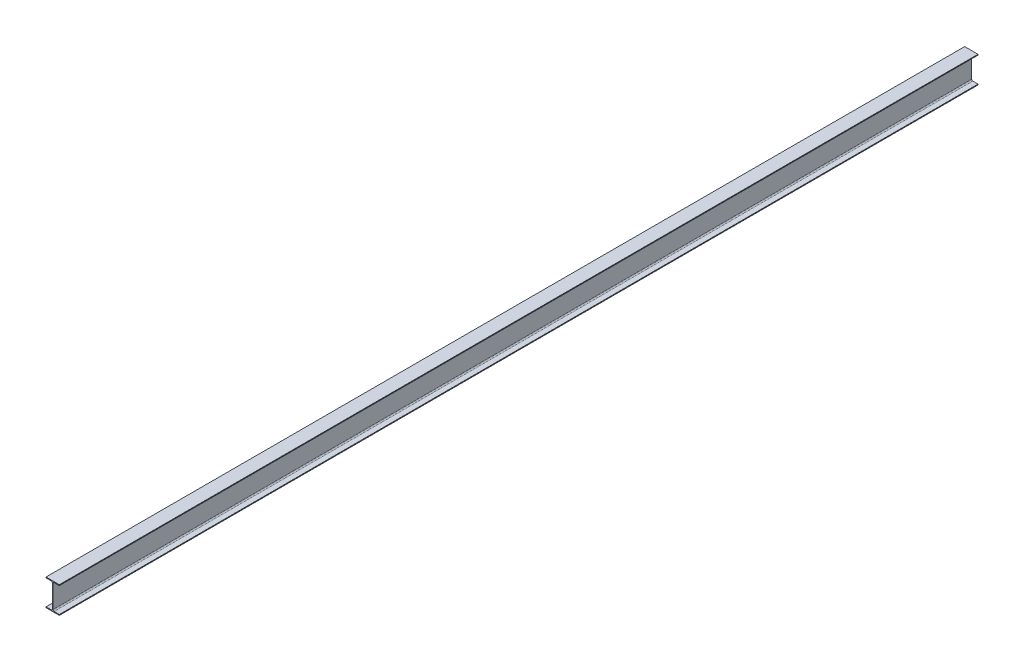
SolidWorks part; units mm, degrees
ref_plane "Front Plane" through (0, 0, 0) normal (0, 0, 1) x (1, 0, 0)
ref_plane "Top Plane" through (0, 0, 0) normal (0, 1, 0) x (1, 0, 0)
ref_plane "Right Plane" through (0, 0, 0) normal (1, 0, 0) x (0, 0, -1)
other "Configuration Table"
sketch "Sketch1" plane through (0, 0, 0) normal (0, 0, 1) x (1, 0, 0)
  line L0 (0, 0) -> (0, 300) construction
  line L1 (75, 0) -> (-75, 0)
  line L2 (-75, 0) -> (-75, 9)
  line L3 (-75, 9) -> (-16.25, 9)
  line L4 (3.25, 22) -> (3.25, 278)
  line L6 (-75, 291) -> (-75, 300)
  line L7 (-75, 300) -> (75, 300)
  line L8 (-3.25, 22) -> (-3.25, 278)
  line L9 (75, 291) -> (75, 300)
  line L10 (16.25, 291) -> (75, 291)
  line L11 (75, 9) -> (16.25, 9)
  line L12 (75, 0) -> (75, 9)
  line L13 (-16.25, 291) -> (-75, 291)
  arc A0 (16.25, 9) -> (3.25, 22) centre (16.25, 22) cw
  arc A1 (-3.25, 22) -> (-16.25, 9) centre (-16.25, 22) cw
  arc A2 (3.25, 278) -> (16.25, 291) centre (16.25, 278) cw
  arc A3 (-3.25, 278) -> (-16.25, 291) centre (-16.25, 278) ccw
  point P18 (3.25, 9)
  point P21 (-3.25, 9)
  point P24 (3.25, 291)
  point P27 (-3.25, 291)
  dimension "D6" = 13
  dimension "D1" = 300
  dimension "D2" = 150
  dimension "D3" = 6.5
  dimension "D4" = 9
  dimension "D5" = 9
extrude "Boss-Extrude1" add sketch "Sketch1" along normal blind 10347
